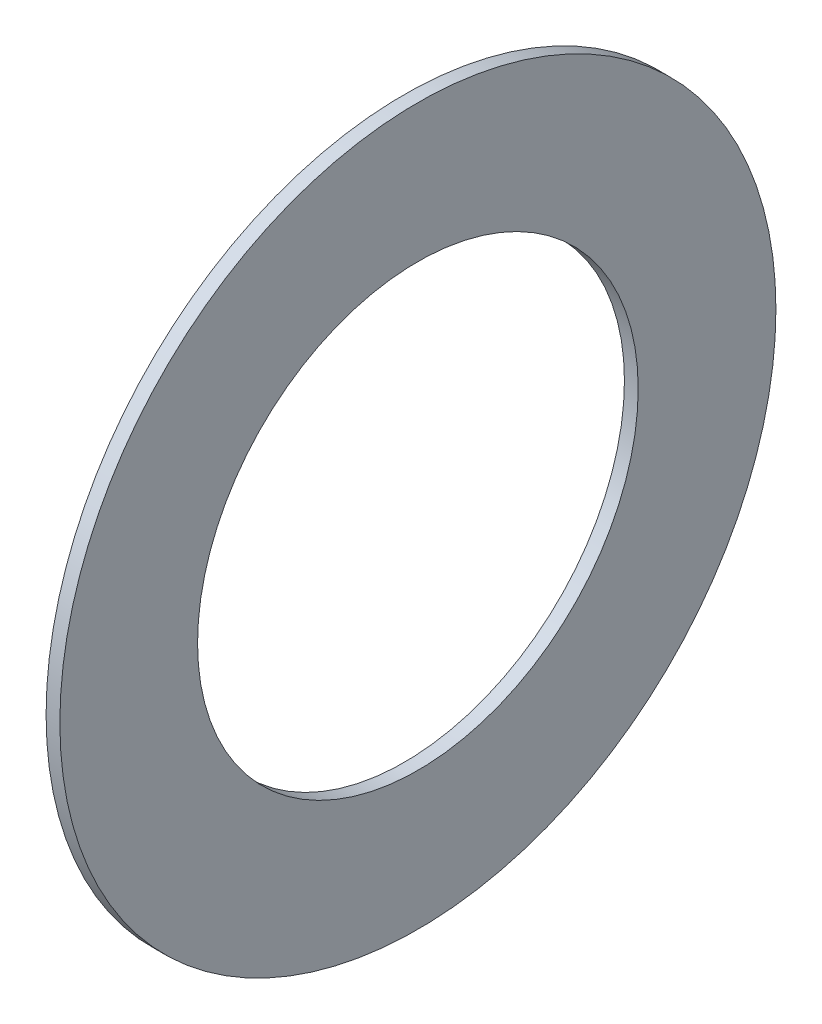
from build123d import *

# Parameters (mm, degrees)
SKETCH1_R           = 13
SKETCH1_R_2         = 8
BOSS_EXTRUDE1_DEPTH = 0.5


with BuildPart() as part:
    # Sketch1 → Boss-Extrude1 (new body)
    with BuildSketch(Plane(origin=(0, 0, 0), x_dir=(0, 0, -1), z_dir=(1, 0, 0))):
        Circle(SKETCH1_R)
        Circle(SKETCH1_R_2, mode=Mode.SUBTRACT)
    extrude(amount=BOSS_EXTRUDE1_DEPTH)


solid = part.part
